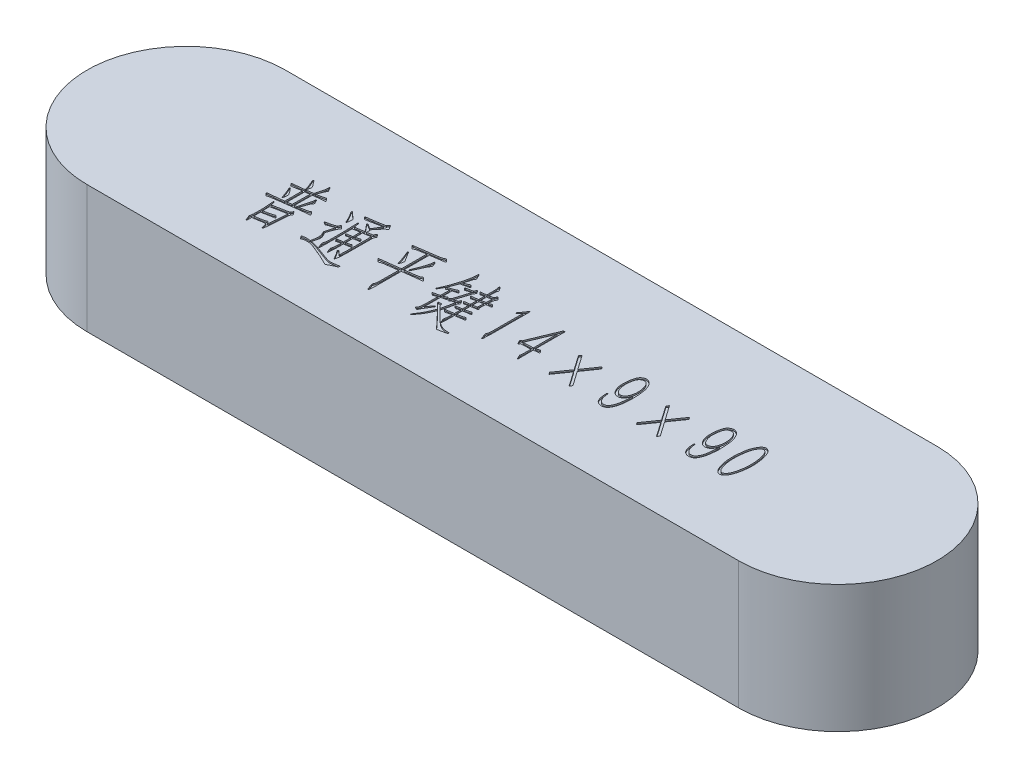
SolidWorks part; units mm, degrees
ref_plane "Front Plane" through (0, 0, 0) normal (0, 0, 1) x (1, 0, 0)
ref_plane "Top Plane" through (0, 0, 0) normal (0, 1, 0) x (1, 0, 0)
ref_plane "Right Plane" through (0, 0, 0) normal (1, 0, 0) x (0, 0, -1)
sketch "Sketch1" plane through (0, 0, 0) normal (0, 1, 0) x (1, 0, 0)
  line L0 (0, 0) -> (46, 0) construction
  line L1 (0, 7) -> (46, 7)
  line L2 (0, -7) -> (46, -7)
  arc A0 (0, 7) -> (0, -7) centre (0, 0) ccw
  arc A1 (46, -7) -> (46, 7) centre (46, 0) ccw
  point P3 (23, 0)
  point P8 (-7, 0)
  point P9 (53, 0)
extrude "Boss-Extrude1" add sketch "Sketch1" along normal blind 9
sketch "Sketch2" plane through (0, 9, 0) normal (0, 1, 0) x (1, 0, 0)
  line L0 (-3.1458, -2.6692) -> (50.6251, -2.6692) construction
  text T0 "普通平键14×9×90" font "汉仪长仿宋体" height 3.5
extrude "Cut-Extrude1" cut sketch "Sketch2" against normal blind 0.1
equation "\"b\"= 14"
equation "\"h\"= 9"
equation "\"l\"= 60"
equation "\"D1@Sketch1\"=\"b\"/2"
equation "\"D2@Sketch1\"=\"l\""
equation "\"D1@Boss-Extrude1\"=\"h\""
